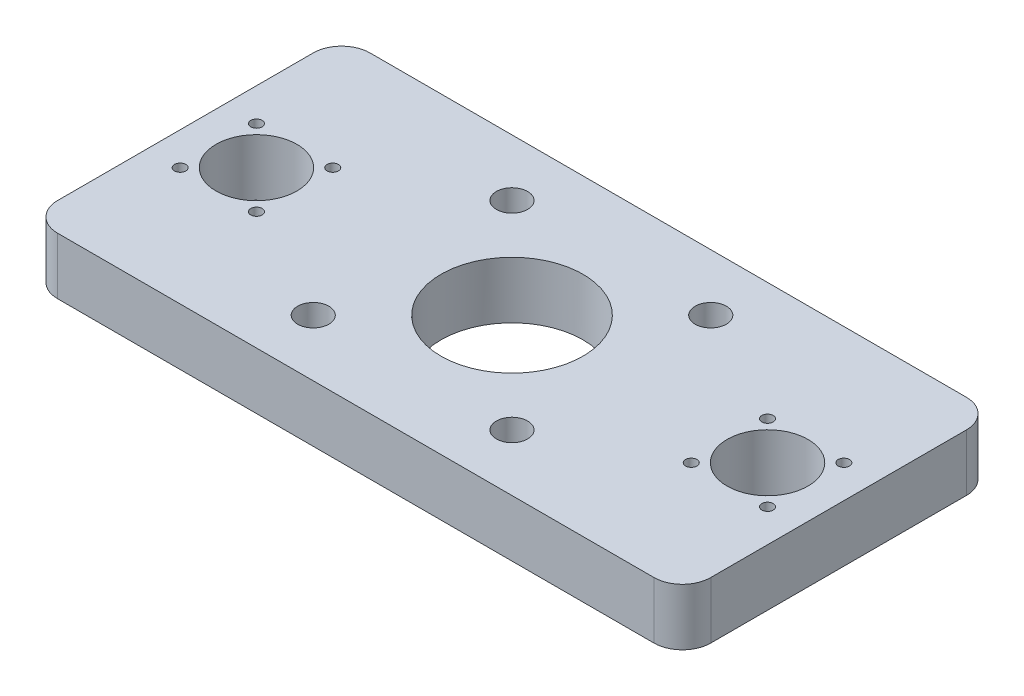
SolidWorks part; units mm, degrees
material "普通碳钢"
ref_plane "Front Plane" through (0, 0, 0) normal (0, 0, 1) x (1, 0, 0)
ref_plane "Top Plane" through (0, 0, 0) normal (0, 1, 0) x (1, 0, 0)
ref_plane "Right Plane" through (0, 0, 0) normal (1, 0, 0) x (0, 0, -1)
sketch "Sketch1" plane through (0, 0, 0) normal (0, 1, 0) x (1, 0, 0)
  line L0 (0, 0) -> (0, 110)
  line L1 (0, 110) -> (230, 110)
  line L2 (230, 110) -> (230, 0)
  line L3 (230, 0) -> (0, 0)
  dimension "D1" = 230
  dimension "D2" = 110
extrude "Boss-Extrude1" add sketch "Sketch1" along normal blind 20
sketch "Sketch2" plane through (0, 20, 0) normal (0, 1, 0) x (1, 0, 0)
  line L0 (25, 55) -> (205, 55) construction
  line L1 (115, 55) -> (115, 0) construction
  line L2 (0, 0) -> (230, 0) construction
  circle A0 centre (25, 55) radius 14.25
  circle A3 centre (205, 55) radius 14.25
  dimension "D1" = 28.5
  dimension "D2" = 180
  dimension "D3" = 55
extrude "Cut-Extrude2" cut sketch "Sketch2" against normal through all
sketch "Sketch3" plane through (0, 20, 0) normal (0, 1, 0) x (1, 0, 0)
  line L0 (11.565, 68.435) -> (25, 55) construction
  line L1 (25, 55) -> (6, 55) construction
  circle A0 centre (25, 55) radius 19 construction
  circle A1 centre (11.565, 68.435) radius 2
  circle A2 centre (38.435, 68.435) radius 2
  circle A3 centre (38.435, 41.565) radius 2
  circle A4 centre (11.565, 41.565) radius 2
  point P15 (25, 55)
  dimension "D1" = 38
  dimension "D3" = 4
  dimension "D2" = 45
  dimension "D4" = 4
extrude "Cut-Extrude3" cut sketch "Sketch3" against normal through all
pattern_linear "LPattern1" count 2 spacing 180 along (1, 0, 0) of "Cut-Extrude3"
pattern_linear "LPattern2" [suppressed] count 2 spacing 70
fillet "Fillet1" radius 10 4 edges at (230, 10, -110) (230, 10, 0) (0, 10, -110) (0, 10, 0)
sketch "Sketch4" plane through (0, 20, 0) normal (0, 1, 0) x (1, 0, 0)
  line L0 (150, 90) -> (150, 20) construction
  line L1 (150, 20) -> (80, 20) construction
  line L2 (80, 20) -> (80, 90) construction
  line L3 (80, 90) -> (150, 90) construction
  line L4 (150, 55) -> (115, 55) construction
  line L5 (115, 55) -> (115, 90) construction
  line L6 (115, 55) -> (115, 0) construction
  line L7 (10, 0) -> (220, 0) construction
  circle A0 centre (115, 55) radius 25
  circle A1 centre (150, 90) radius 5.5
  circle A2 centre (150, 20) radius 5.5
  circle A3 centre (80, 20) radius 5.5
  circle A4 centre (80, 90) radius 5.5
  dimension "D4" = 11
  dimension "D5" = 50
  dimension "D1" = 70
  dimension "D2" = 70
  dimension "D3" = 55
extrude "Cut-Extrude4" cut sketch "Sketch4" against normal blind 100
hole_wizard "M12 Tapped Hole1" positions "Sketch5" profile "Sketch6" tap size "M12" standard "GB"
sketch "Sketch5" plane through (0, 0, -110) normal (0, 0, -1) x (-1, 0, 0)
  line L0 (-220, 12.5) -> (-190, 12.5) construction
  line L1 (-220, 25) -> (-220, 0) construction
  line L2 (-190, 12.5) -> (-140, 12.5) construction
  line L3 (-140, 12.5) -> (-90, 12.5) construction
  line L4 (-90, 12.5) -> (-40, 12.5) construction
  line L6 (-115, 12.5) -> (-115, 0) construction
  line L7 (-220, 0) -> (-10, 0) construction
  point P0 (-190, 12.5)
  point P2 (-140, 12.5)
  point P4 (-90, 12.5)
  point P6 (-40, 12.5)
  dimension "D1" = 50
sketch "Sketch6" plane through (190, 12.5, -110) normal (1, 0, 0) x (0, 1, 0)
  line L0 (0, 0) -> (0, 32.3144)
  line L1 (0, 32.3144) -> (5.1, 29.25)
  line L2 (5.1, 29.25) -> (5.1, 0)
  line L5 (5.1, 0) -> (0, 0)
  line L10 (0, 32.3144) -> (-5.1, 29.25) construction
  line L11 (0, -6.35) -> (0, 107.95) construction
  dimension "螺纹孔钻头直径" = 10.2
  dimension "螺纹孔钻头深度" = 29.25
  dimension "导头角度" = 118
cosmetic thread "Hole Thread1" [suppressed] parameters "D1"=24, "D2"=12
cosmetic thread "Hole Thread2" [suppressed] parameters "D1"=24, "D2"=12
cosmetic thread "Hole Thread3" [suppressed] parameters "D1"=24, "D2"=12
cosmetic thread "Hole Thread4" [suppressed] parameters "D1"=24, "D2"=12
hole_wizard "M12 Tapped Hole2" positions "Sketch7" profile "Sketch8" tap size "M12" standard "GB"
sketch "Sketch7" plane through (0, 0, -110) normal (0, 0, -1) x (-1, 0, 0)
  line L0 (-220, 10) -> (-200, 10) construction
  line L1 (-220, 20) -> (-220, 0) construction
  line L2 (-200, 10) -> (-115, 10) construction
  line L3 (-115, 10) -> (-30, 10) construction
  line L5 (-115, 10) -> (-115, 0) construction
  line L6 (-220, 0) -> (-10, 0) construction
  point P0 (-200, 10)
  point P2 (-115, 10)
  point P4 (-30, 10)
  dimension "D1" = 85
sketch "Sketch8" plane through (200, 10, -110) normal (1, 0, 0) x (0, 1, 0)
  line L0 (0, 0) -> (0, 23.0644)
  line L1 (0, 23.0644) -> (5.1, 20)
  line L2 (5.1, 20) -> (5.1, 0)
  line L5 (5.1, 0) -> (0, 0)
  line L10 (0, 23.0644) -> (-5.1, 20) construction
  line L11 (0, -6.35) -> (0, 107.95) construction
  dimension "螺纹孔钻头直径" = 10.2
  dimension "螺纹孔钻头深度" = 20
  dimension "导头角度" = 118
cosmetic thread "Hole Thread5" parameters "D1"=24, "D2"=12
cosmetic thread "Hole Thread6" parameters "D1"=24, "D2"=12
cosmetic thread "Hole Thread7" parameters "D1"=24, "D2"=12
